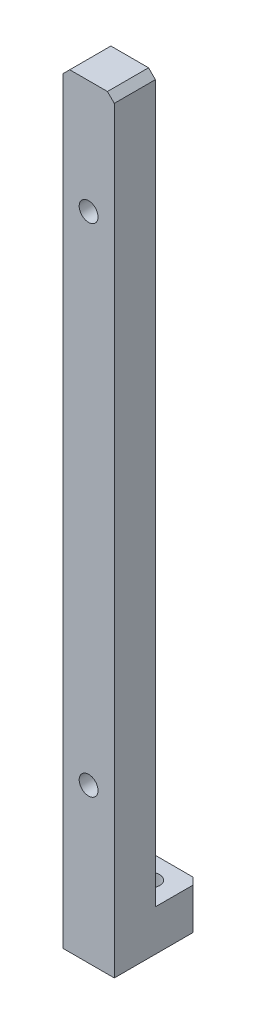
from build123d import *

# Parameters (mm, degrees)
BOSS_EXTRUDE1_DEPTH                                  = 15
CBORE_FOR_M5_HEXAGON_SOCKET_HEAD_CAP_SCR_D           = 5.5
CBORE_FOR_M5_HEXAGON_SOCKET_HEAD_CAP_SCR_CBORE_D     = 10
CBORE_FOR_M5_HEXAGON_SOCKET_HEAD_CAP_SCR_CBORE_DEPTH = 5.7
M5_CLEARANCE_HOLE1_D                                 = 5.5
CHAMFER1_SIZE                                        = 2


with BuildPart() as part:
    # Sketch1 → Boss-Extrude1 (new body)
    with BuildSketch(Plane(origin=(0, 0, 0), x_dir=(0, 0, -1), z_dir=(1, 0, 0))):
        Polygon((0, 0), (25, 0), (25, 12), (12, 12), (12, 223.1), (0, 223.1), align=None)
    extrude(amount=BOSS_EXTRUDE1_DEPTH)

    # CBORE for M5 Hexagon socket head cap screws1 (through all)
    with Locations(Plane(origin=(0, 0, -12), x_dir=(-1, 0, 0), z_dir=(0, 0, -1))):
        with Locations((-7.5, 45), (-7.5, 190)):
            CounterBoreHole(CBORE_FOR_M5_HEXAGON_SOCKET_HEAD_CAP_SCR_D / 2, CBORE_FOR_M5_HEXAGON_SOCKET_HEAD_CAP_SCR_CBORE_D / 2, CBORE_FOR_M5_HEXAGON_SOCKET_HEAD_CAP_SCR_CBORE_DEPTH)

    # M5 Clearance Hole1 (through all)
    with Locations(Plane(origin=(0, 0, 0), x_dir=(-1, 0, 0), z_dir=(0, -1, 0))):
        with Locations((-7.5, 18)):
            Hole(M5_CLEARANCE_HOLE1_D / 2)

    # Chamfer1
    chamfer1_edges = [part.edges().sort_by_distance(p)[0] for p in [
        (15, 6, -25),
        (15, 223.1, -6),
        (0, 223.1, -6),
        (0, 6, -25),
    ]]
    chamfer(chamfer1_edges, length=CHAMFER1_SIZE)


solid = part.part
